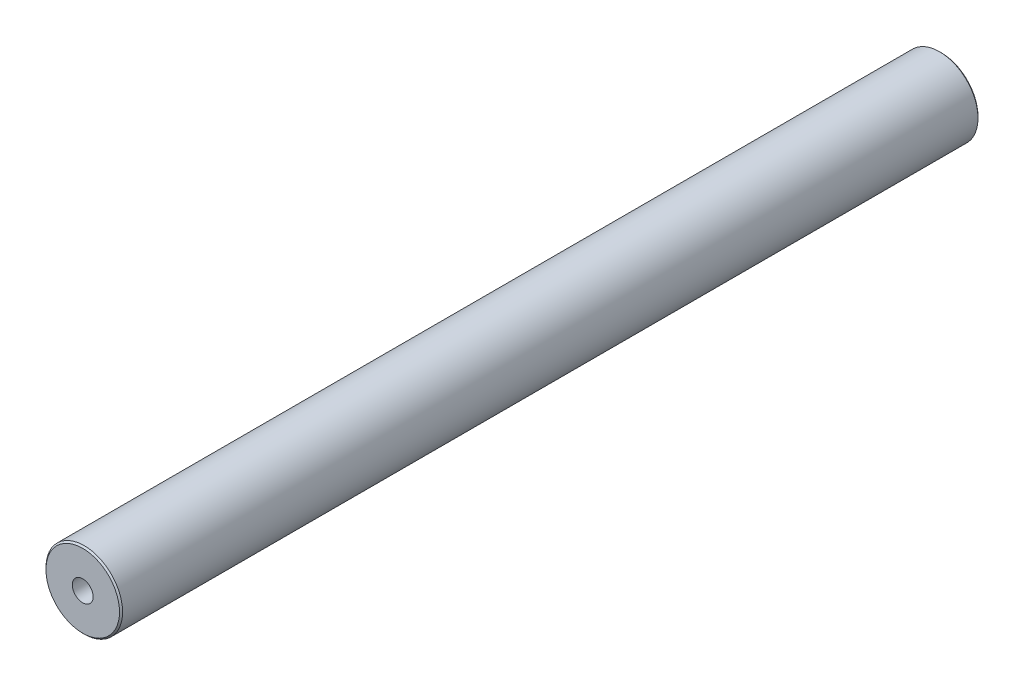
SolidWorks part; units mm, degrees
ref_plane "前视基准面" through (0, 0, 0) normal (0, 0, 1) x (1, 0, 0)
ref_plane "上视基准面" through (0, 0, 0) normal (0, 1, 0) x (1, 0, 0)
ref_plane "右视基准面" through (0, 0, 0) normal (1, 0, 0) x (0, 0, -1)
sketch "草图1" plane through (0, 0, 0) normal (0, 0, 1) x (1, 0, 0)
  circle A0 centre (0, 0) radius 12.5
  dimension "D1" = 25
extrude "凸台-拉伸1" add sketch "草图1" along normal blind 280
hole_wizard "M8 螺纹孔1" positions "草图3" profile "草图4" tap size "M8" standard "ISO"
sketch "草图3" plane through (0, 0, 280) normal (0, 0, 1) x (1, 0, 0)
  point P0 (0, 0)
sketch "草图4" plane through (0, 0, 280) normal (1, 0, 0) x (0, -1, 0)
  line L0 (0, 0) -> (0, 24.2929)
  line L1 (0, 24.2929) -> (3.4, 22.25)
  line L2 (3.4, 22.25) -> (3.4, 0)
  line L5 (3.4, 0) -> (0, 0)
  line L10 (0, 24.2929) -> (-3.4, 22.25) construction
  line L11 (0, -6.35) -> (0, 107.95) construction
  dimension "螺纹孔钻头直径" = 6.8
  dimension "螺纹孔钻头深度" = 22.25
  dimension "导头角度" = 118
cosmetic thread "孔螺蚊线1"
hole_wizard "M8 螺纹孔2" positions "草图6" profile "草图5" tap size "M8" standard "ISO"
sketch "草图6" plane through (0, 0, 0) normal (0, 0, -1) x (-1, 0, 0)
  point P0 (0, 0)
sketch "草图5" plane through (0, 0, 0) normal (1, 0, 0) x (0, 1, 0)
  line L0 (0, 0) -> (0, 24.2929)
  line L1 (0, 24.2929) -> (3.4, 22.25)
  line L2 (3.4, 22.25) -> (3.4, 0)
  line L5 (3.4, 0) -> (0, 0)
  line L10 (0, 24.2929) -> (-3.4, 22.25) construction
  line L11 (0, -6.35) -> (0, 107.95) construction
  dimension "螺纹孔钻头直径" = 6.8
  dimension "螺纹孔钻头深度" = 22.25
  dimension "导头角度" = 118
cosmetic thread "孔螺蚊线2" parameters "D1"=16, "D2"=8
chamfer "倒角1" distance 0.5 angle 45 2 edges at (12.5, 0, 280) (12.5, 0, 0)
